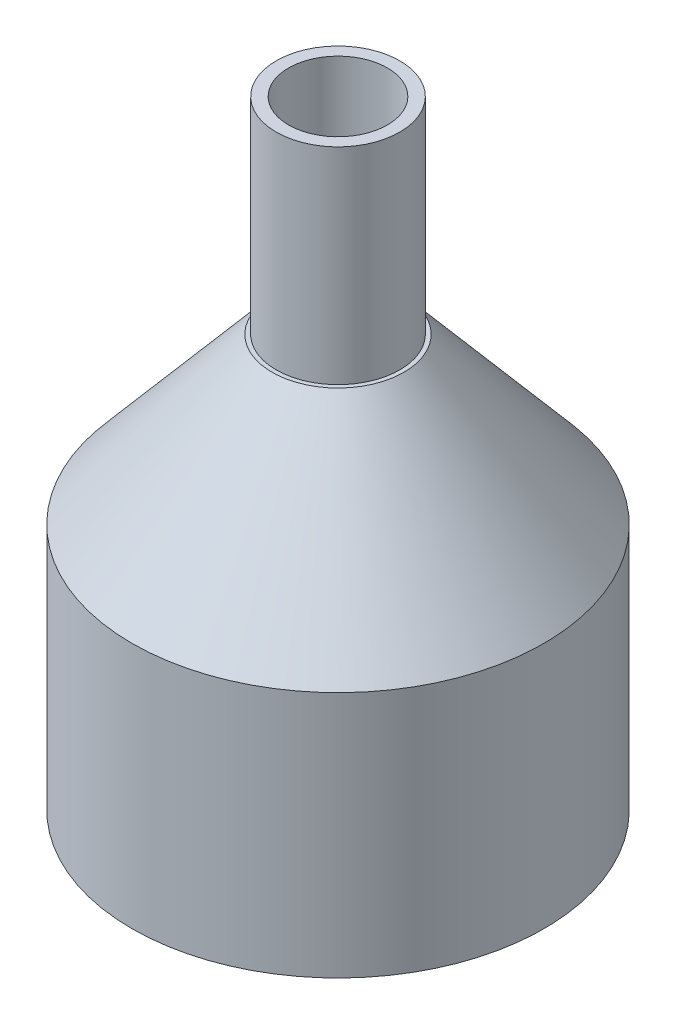
from build123d import *

# Parameters (mm, degrees)
SKETCH1_R           = 25
BOSS_EXTRUDE1_DEPTH = 50
SKETCH2_R           = 7.5
BOSS_EXTRUDE2_DEPTH = 25
CHAMFER1_SIZE       = 20
CHAMFER1_SIZE2      = 17
SKETCH3_R           = 6
CUT_EXTRUDE1_DEPTH  = 83.915619759
SKETCH4_R           = 21.453348456
CUT_EXTRUDE2_DEPTH  = 15


with BuildPart() as part:
    # Sketch1 → Boss-Extrude1 (new body)
    with BuildSketch(Plane(origin=(0, 0, 0), x_dir=(1, 0, 0), z_dir=(0, 1, 0))):
        with Locations(Location((0, 0, 0), (0, 0, 270))):
            Circle(SKETCH1_R)
    extrude(amount=BOSS_EXTRUDE1_DEPTH)

    # Sketch2 → Boss-Extrude2 (add)
    with BuildSketch(Plane(origin=(0, 50, 0), x_dir=(1, 0, 0), z_dir=(0, 1, 0))):
        with Locations(Location((0, 0, 0), (0, 0, 270))):
            Circle(SKETCH2_R)
    extrude(amount=BOSS_EXTRUDE2_DEPTH)

    # Chamfer1
    chamfer1_edges = [part.edges().sort_by_distance(p)[0] for p in [
        (0, 50, -25),
    ]]
    chamfer1_side = [part.faces().sort_by_distance(p)[0] for p in [
        (0, 25, -25),
    ]]
    chamfer(chamfer1_edges, length=CHAMFER1_SIZE, length2=CHAMFER1_SIZE2, reference=chamfer1_side[0])

    # Sketch3 → Cut-Extrude1 (cut, through all)
    with BuildSketch(Plane(origin=(0, 75, 0), x_dir=(1, 0, 0), z_dir=(0, 1, 0))):
        with Locations(Location((0, 0, 0), (0, 0, 270))):
            Circle(SKETCH3_R)
    extrude(amount=-CUT_EXTRUDE1_DEPTH, mode=Mode.SUBTRACT)

    # Sketch4 → Cut-Extrude2 (cut)
    with BuildSketch(Plane.XZ):
        with Locations(Location((0, 0, 0), (0, 0, 270))):
            Circle(SKETCH4_R)
    extrude(amount=-CUT_EXTRUDE2_DEPTH, mode=Mode.SUBTRACT)


solid = part.part
